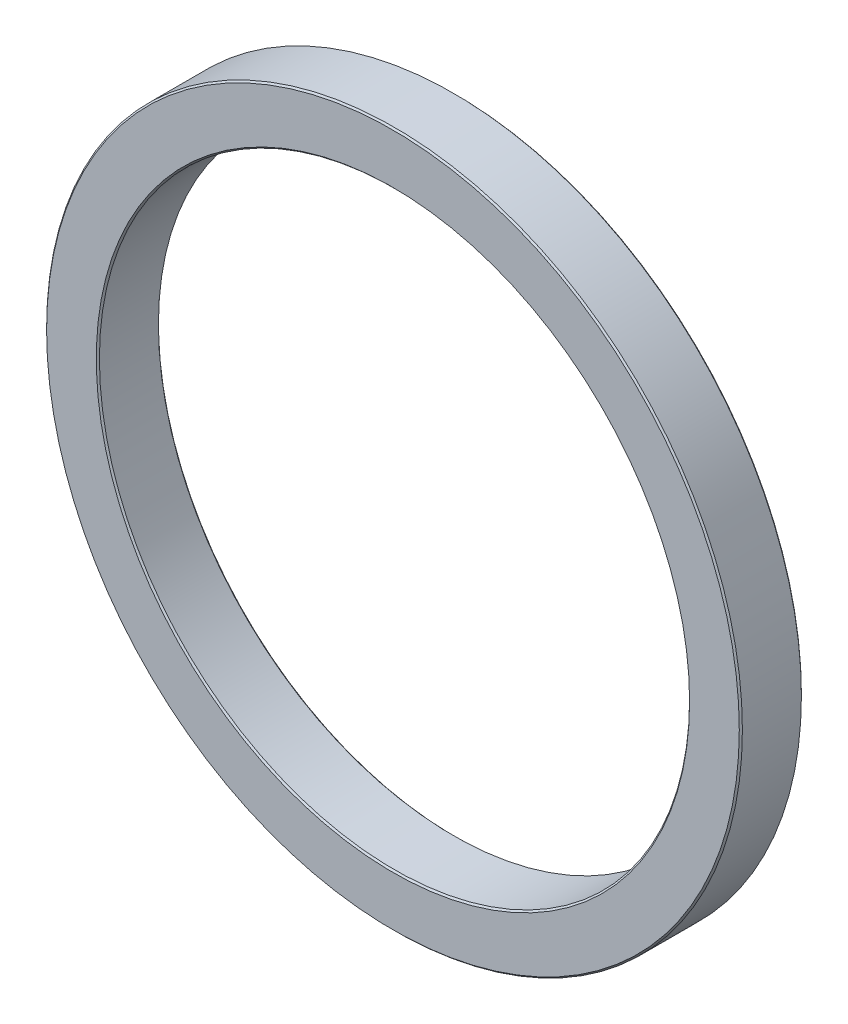
from build123d import *

# Parameters (mm, degrees)
SKETCH_1_R             = 56
SKETCH_1_R_2           = 47.5
EXTRUDE_1_DEPTH        = 10
HOLE_WIZARD_M4_1_D     = 3.3
HOLE_WIZARD_M4_1_DEPTH = 7.5
CHAMFER_1_SIZE         = 0.25
SKETCH_5_R             = 50
SKETCH_5_R_2           = 48.5
CUT_EXTRUDE_1_DEPTH    = 1.2


with BuildPart() as part:
    # 草图1 → 凸台-拉伸1 (new body)
    with BuildSketch(Plane.XY):
        Circle(SKETCH_1_R)
        Circle(SKETCH_1_R_2, mode=Mode.SUBTRACT)
    extrude(amount=EXTRUDE_1_DEPTH)

    # M4 螺纹孔1
    with Locations(Plane(origin=(0, 0, 0), x_dir=(-1, 0, 0), z_dir=(0, 0, -1))):
        with Locations((35.5, 0), (0, 35.5), (0, -35.5), (-35.5, 0), (-37.476659403, -37.476659403), (37.476659403, -37.476659403), (37.476659403, 37.476659403), (-37.476659403, 37.476659403), (0, 53), (53, 0), (0, -53), (-53, 0)):
            Hole(HOLE_WIZARD_M4_1_D / 2, depth=HOLE_WIZARD_M4_1_DEPTH)

    # 倒角1
    chamfer_1_edges = [part.edges().sort_by_distance(p)[0] for p in [
        (-56, 0, 0),
        (-56, 0, 10),
        (-47.5, 0, 0),
        (-47.5, 0, 10),
    ]]
    chamfer(chamfer_1_edges, length=CHAMFER_1_SIZE)

    # 草图5 → 切除-拉伸1 (cut)
    with BuildSketch(Plane(origin=(0, 0, 0), x_dir=(-1, 0, 0), z_dir=(0, 0, -1))):
        Circle(SKETCH_5_R)
        Circle(SKETCH_5_R_2, mode=Mode.SUBTRACT)
    extrude(amount=-CUT_EXTRUDE_1_DEPTH, mode=Mode.SUBTRACT)


solid = part.part
